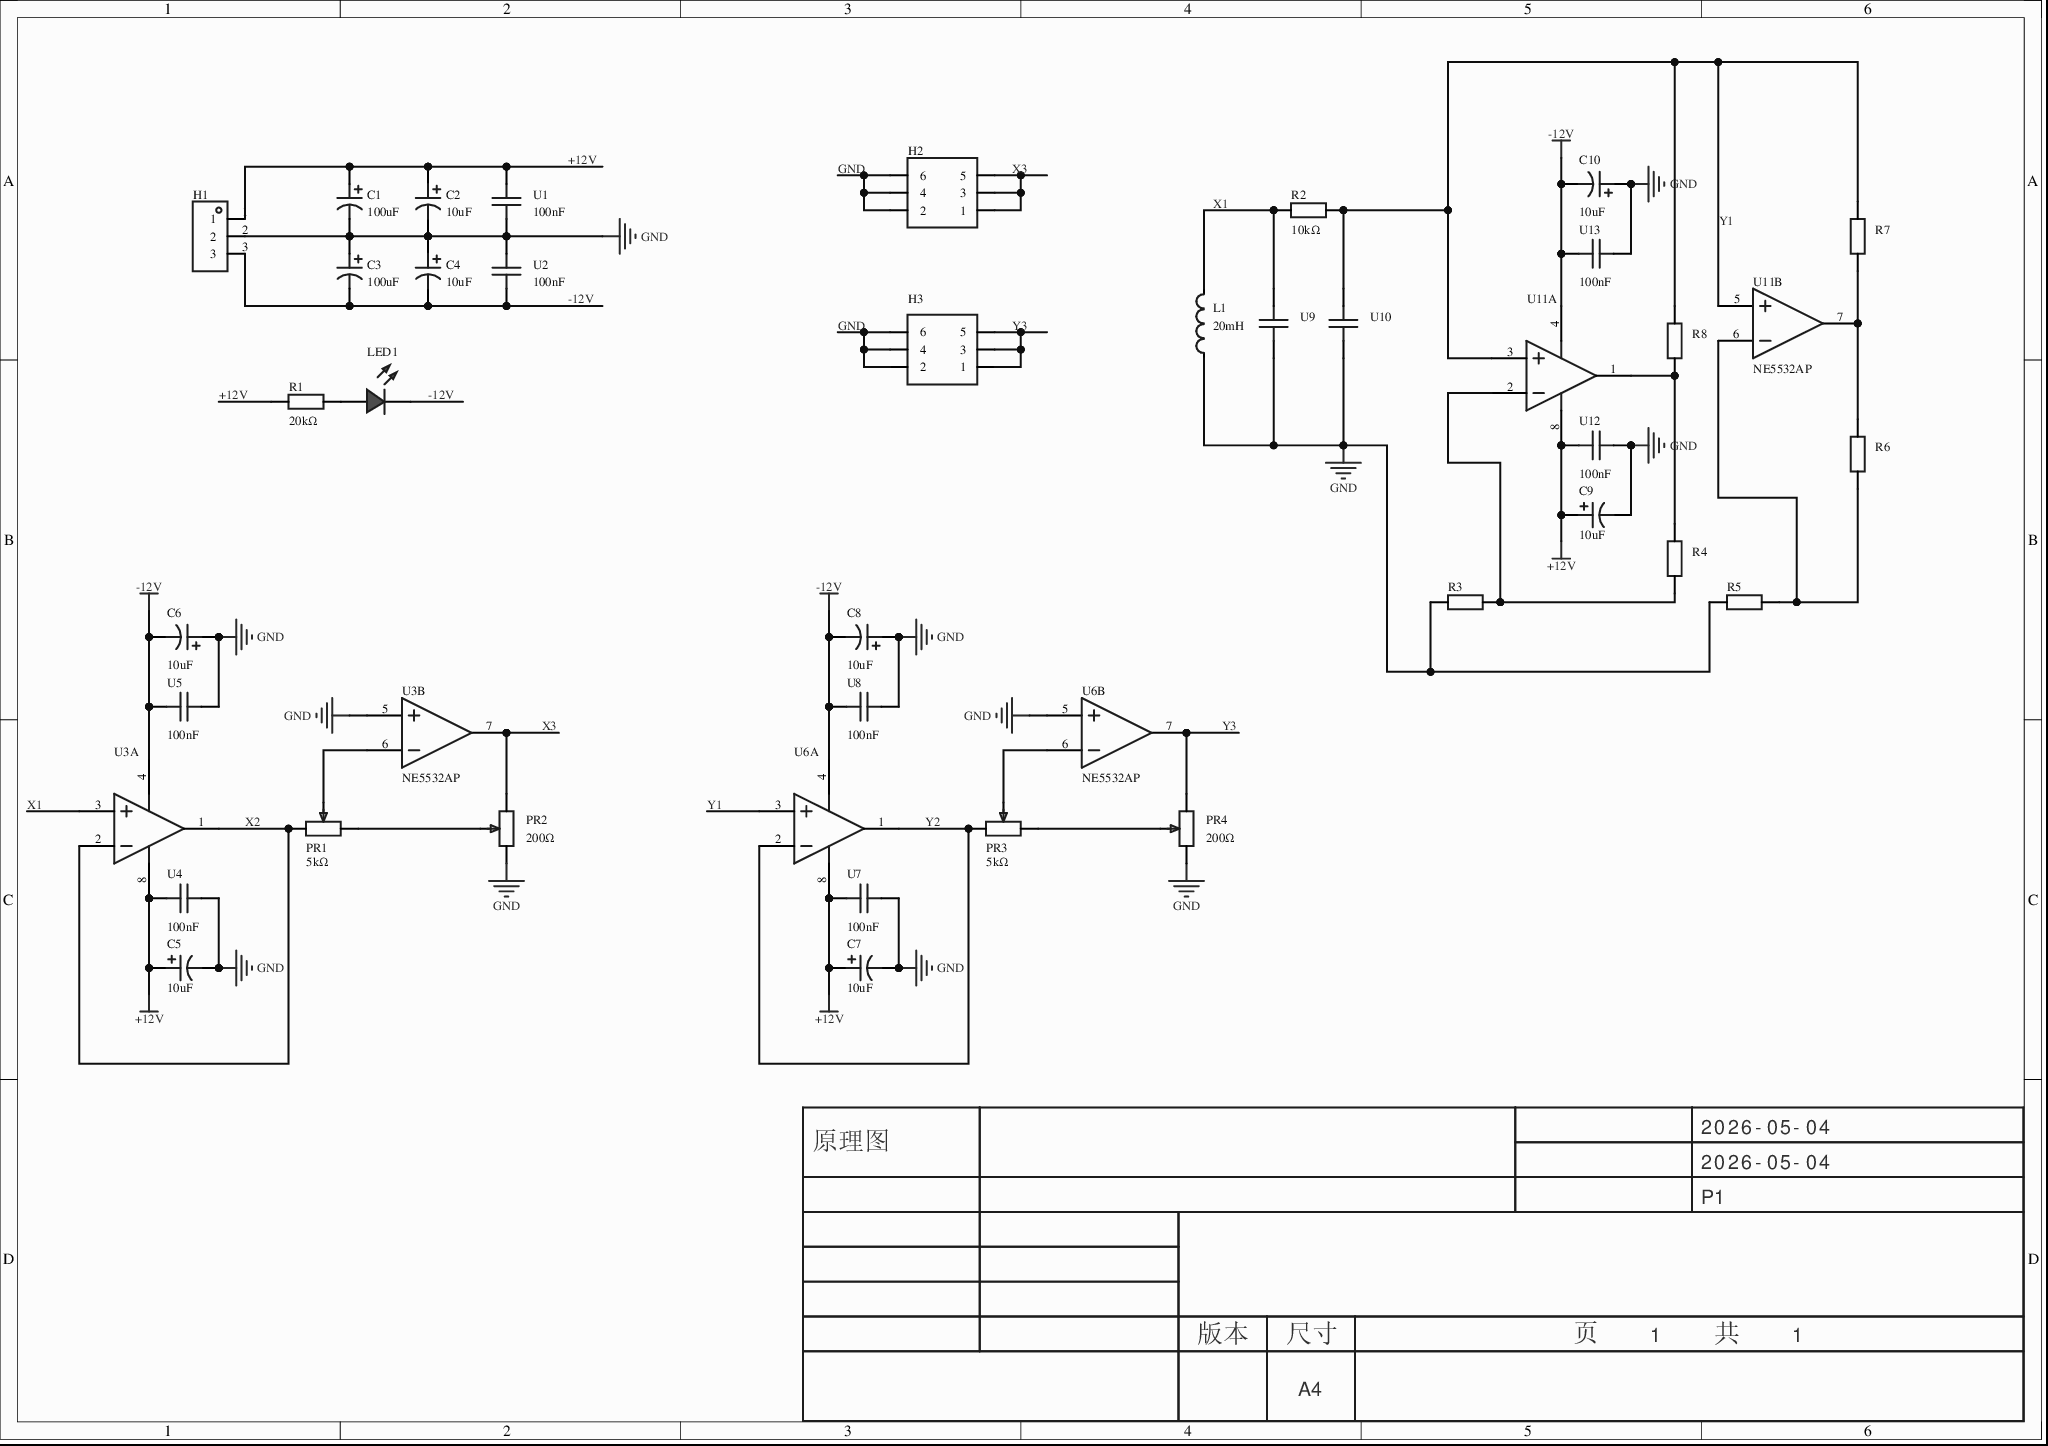
[diagram p0: MISC51743-3.schdoc]
# Altium project MISC51743-2.PrjPcb
1 sheet, 40 parts. Net scope: global (net labels, ports and power ports of the same name join across sheets).
Board file: MISC51743.pcbdoc

## Sheet MISC51743-3.schdoc
size 297 x 209 mm; Version: V1.0; @Project Name: MISC51743; @Update Date: 2026-05-04; @Create Date: 2026-05-04; @Board Name: MISC51743; @Create Time: 17:21:46; @Page Count: 1; @Page No: 1; @Schematic Name: MISC51743; @Update Time: 17:21:46; Size: A4

### Parts
C1  100uF  [CAP-TH_BD8.0-P3.50-D0.6-FD_1]
C2  10uF  [CAP-TH_BD5.0-P2.00-D0.8-FD-10UF50VC110GL]
C3  100uF  [CAP-TH_BD8.0-P3.50-D0.6-FD_1]
C4  10uF  [CAP-TH_BD5.0-P2.00-D0.8-FD-10UF50VC110GL]
C5  10uF  [CAP-TH_BD5.0-P2.00-D0.8-FD-10UF50VC110GL]
C6  10uF  [CAP-TH_BD5.0-P2.00-D0.8-FD-10UF50VC110GL]
C7  10uF  [CAP-TH_BD5.0-P2.00-D0.8-FD-10UF50VC110GL]
C8  10uF  [CAP-TH_BD5.0-P2.00-D0.8-FD-10UF50VC110GL]
C9  10uF  [CAP-TH_BD5.0-P2.00-D0.8-FD-10UF50VC110GL]
C10  10uF  [CAP-TH_BD5.0-P2.00-D0.8-FD-10UF50VC110GL]
H1  (no value)  [HDR-TH_3P-P2.54-V-M]
H2  (no value)  [HDR-TH_6P-P2.54-V-F-R2-C3-S2.54]
H3  (no value)  [HDR-TH_6P-P2.54-V-F-R2-C3-S2.54]
L1  20mH  [L0603]
LED1  (no value)  [LED_TH-3mm]
PR1  5kΩ  [R_3296]
PR2  200Ω  [R_3296]
PR3  5kΩ  [R_3296]
PR4  200Ω  [R_3296]
R1  20kΩ  [Res_1/8W]
R2  10kΩ  [Res_1/8W]
R3  10kΩ  [Res_1/8W]  (value not drawn)
R4  10kΩ  [Res_1/8W]  (value not drawn)
R5  10kΩ  [Res_1/8W]  (value not drawn)
R6  10kΩ  [Res_1/8W]  (value not drawn)
R7  10kΩ  [Res_1/8W]  (value not drawn)
R8  10kΩ  [Res_1/8W]  (value not drawn)
U1  100nF  [CAP-TH_L5.0-W2.5-P5.00-D1.0]
U2  100nF  [CAP-TH_L5.0-W2.5-P5.00-D1.0]
U3  NE5532AP  [PDIP-8_L9.6-W6.4-P2.54-LS7.6-BL]  (value not drawn)  (parts A,B of 2)
U4  100nF  [CAP-TH_L5.0-W2.5-P5.00-D1.0]
U5  100nF  [CAP-TH_L5.0-W2.5-P5.00-D1.0]
U6  NE5532AP  [PDIP-8_L9.6-W6.4-P2.54-LS7.6-BL]  (value not drawn)  (parts A,B of 2)
U7  100nF  [CAP-TH_L5.0-W2.5-P5.00-D1.0]
U8  100nF  [CAP-TH_L5.0-W2.5-P5.00-D1.0]
U9  100nF  [CAP-TH_L5.0-W2.5-P5.00-D1.0]  (value not drawn)
U10  100nF  [CAP-TH_L5.0-W2.5-P5.00-D1.0]  (value not drawn)
U11  NE5532AP  [PDIP-8_L9.6-W6.4-P2.54-LS7.6-BL]  (value not drawn)  (parts A,B of 2)
U12  100nF  [CAP-TH_L5.0-W2.5-P5.00-D1.0]
U13  100nF  [CAP-TH_L5.0-W2.5-P5.00-D1.0]

### Nets
+12V: C1.1 C2.1 C5.1 C7.1 C9.1 H1.1 R1.1 U1.1 U3.8(V+) U4.2 U6.8(V+) U7.2 U11.8(V+) U12.2
-12V: C3.2 C4.2 C6.2 C8.2 C10.2 H1.3 LED1.2(A) U2.2 U3.4(V-) U5.2 U6.4(V-) U8.2 U11.4(V-) U13.2
GND: C1.2 C2.2 C3.1 C4.1 C5.2 C6.1 C7.2 C8.1 C9.2 C10.1 H1.2 H2.2 H2.4 H2.6 H3.2 H3.4 H3.6 L1.1 PR2.3 PR4.3 R3.1 R5.1 U1.2 U2.1 U3.5(IN_B+) U4.1 U5.1 U6.5(IN_B+) U7.1 U8.1 U9.2 U10.2 U12.1 U13.1
X1: L1.2 R2.1 U3.3(IN_A+) U9.1
X2: PR1.3 U3.1(OUT_A) U3.2(IN_A-)
X3: H2.1 H2.3 H2.5 PR2.1 U3.7(OUT_B)
Y1: R2.2 R7.2 R8.2 U6.3(IN_A+) U10.1 U11.3(IN_A+) U11.5(IN_B+)
Y2: PR3.3 U6.1(OUT_A) U6.2(IN_A-)
Y3: H3.1 H3.3 H3.5 PR4.1 U6.7(OUT_B)
NetLED1_1: LED1.1(C) R1.2
NetPR1_1: PR1.1 PR2.2
NetPR1_2: PR1.2 U3.6(IN_B-)
NetPR3_1: PR3.1 PR4.2
NetPR3_2: PR3.2 U6.6(IN_B-)
NetR3_2: R3.2 R4.1 U11.2(IN_A-)
NetR4_2: R4.2 R8.1 U11.1(OUT_A)
NetR5_2: R5.2 R6.1 U11.6(IN_B-)
NetR6_2: R6.2 R7.1 U11.7(OUT_B)

### Notes on the sheet
- 2026-05-04
- 原理图
- P1
- 版本
- 尺寸
- A4
- 页    1    共    1

### Library data of the parts
C1 C3 = 100uF: Symbol: 100UF_C9900016884; AddInBom: yes; ModelId: 5fc21599cab34df2ad7753b19b2f52860819f05c4eef4c71ace90d822a990e87; ModelTransform: 315.365,314.914,0,0,0,0,0,0,-196.85; Device: 100uF; LCSC Part Name: 100uF; SupplierPart: C9900016884; ManufacturerPart: 100uF; Supplier Footprint: CAP-TH_BD8.0-P3.50-D1.0-FD; JLCPCB Part Class: Extended Part; Supplier: LCSC; ConvertToPcb: yes; FootprintName: CAP-TH_BD8.0-P3.50-D0.6-FD_1; ModelName: CAP-TH_BD8.0-P3.50-D0.6-FD_1
C2 C4-C10 = 10UF50VC110GL: 容值:10uF;精度:±20%;额定电压:50V;纹波电流:120mA@100KHz;等效串联电阻(ESR):1.6Ω;; Manufacturer: Econd(米朗电子); AddInBom: yes; Tolerance: ±20%; Voltage Rating: 50V; Equivalent Series Resistance(ESR): 1.6Ω; Pin Spacing: 2mm; Lifetime: 5000hrs@105℃; Symbol: 10UF50VC110GL; Device: 10UF50VC110GL; LCSC Part Name: 10uF ±20% 50V; SupplierPart: C46867109; ManufacturerPart: 10UF50VC110GL; Supplier Footprint: 插件,D5xL11mm; JLCPCB Part Class: Extended Part; Datasheet: https://item.szlcsc.com/datasheet/10UF50VC110GL/49031974.html; Supplier: LCSC; ConvertToPcb: yes; FootprintName: CAP-TH_BD5.0-P2.00-D0.8-FD-10UF50VC110GL; Value: 10uF; Ripple Current: 120mA@100KHz; Diameter: 5mm; Height - Seated (Max): 11mm; Operating Temperature: -40℃~+105℃
H1 = HDR-M_2.54_1x3P: AddInBom: yes; ModelId: bb473b6d38ff42a99216a4fcdbdcc4cb0819f05c4eef4c71ace90d822a990e87; ModelName: HDR-TH_3P-P2.54-M-LI-1X3P; ModelTransform: 300.03877,100,0,0,0,0,0,0,-118.11; Symbol: HDR-M_2.54_1x3P; Device: HDR-M_2.54_1x3P; ConvertToPcb: yes; FootprintName: HDR-TH_3P-P2.54-V-M; SupplierPart: C2937625; Supplier Footprint: 插件
H2 H3 = HDR-F_2.54_2x3: Symbol: HDR-F-2.54_2x3; ConvertToPcb: yes; ModelId: 6dbaf143e10146ae9674d03402f6f9fb0819f05c4eef4c71ace90d822a990e87; ModelName: HDR-TH_6P-P2.54-F-LI-2X3P; ModelTransform: 315.7474,196.85,0,0,0,0,0,0,-125.984; Device: HDR-F_2.54_2x3; AddInBom: yes; SupplierPart: C92272; Supplier Footprint: 插件; FootprintName: HDR-TH_6P-P2.54-V-F-R2-C3-S2.54
L1 = L_0603: Symbol: SDFL1608S100KTF; AddInBom: yes; ModelId: 2bc5ec593d464d6ba9807aec0b5673c20819f05c4eef4c71ace90d822a990e87; ModelName: L0603_L1.6-W0.8-H0.5_BEAD; ModelTransform: 62.992,31.496,0,180,0,0,0.094,0.629,0; Device: L_0603; Value: 20mH; Supplier Footprint: L0603; ConvertToPcb: yes; FootprintName: L0603
LED1 = LED_TH-R_3mm: ConvertToPcb: yes; ModelId: a497c992633541038a38947cdc58012f0819f05c4eef4c71ace90d822a990e87; ModelName: LED-TH-3mm_R; ModelTransform: 141.274,153.327,0,0,0,0,-5.984,0,-137.795; Symbol: LED_TH-R; Device: LED_TH-R_3mm; AddInBom: yes; FootprintName: LED_TH-3mm; Supplier Footprint: 插件
PR1-PR4 = R_3296: ConvertToPcb: yes; ModelId: b182808559bb43bda9e7de64b64134cb0819f05c4eef4c71ace90d822a990e87; ModelName: 3296W; ModelTransform: 373.98,188.96,590.49,180,0,0,0,0,-140; Symbol: R_3296; Device: R_3296; AddInBom: yes; Supplier Footprint: 直插; FootprintName: R_3296
  PR1 PR3: Value: 5kΩ
  PR2 PR4: Value: 200Ω
R1-R8 = Res_AXIAL-1/8W: Symbol: 电阻; ConvertToPcb: yes; ModelId: b2b5ae7ae4c642178fe0039925c86a3f0819f05c4eef4c71ace90d822a990e87; ModelName: RES-TH_BD1.8-L3.2-P7.20-D0.4; ModelTransform: 282.86,66.88,253.09,0,0,0,0,0,-191; Device: Res_AXIAL-1/8W; AddInBom: yes; Supplier Footprint: 轴向引线; FootprintName: Res_1/8W
  R1: Value: 20kΩ
  R2-R8: Value: 10kΩ
U1 U2 U4 U5 U7-U10 U12 U13 = 100nF: Symbol: 100NF_C9900015256; AddInBom: yes; ModelId: 08e3d7481fc7486bb1b263873f51e1e10819f05c4eef4c71ace90d822a990e87; ModelName: CAP-TH_BD5.0-W2.5-P5.08; ModelTransform: 224.652,98.425,0,0,0,0,-0.005,0,-137.795; Device: 100nF; LCSC Part Name: 100nF; SupplierPart: C9900015256; ManufacturerPart: 100nF; Supplier Footprint: CAP-TH_L5.0-W2.5-P5.00-D1.0; JLCPCB Part Class: Extended Part; Supplier: LCSC; ConvertToPcb: yes; FootprintName: CAP-TH_L5.0-W2.5-P5.00-D1.0
U3 U6 U11 = NE5532AP: NE5532A 适用于音频应用的双通道、30V、10MHz、低噪声 (6nV/√Hz) 运算放大器; Manufacturer: TI(德州仪器); Relevance: []; AddInBom: yes; ModelId: 5dc2af053da0476fab11ee64b9a10a940819f05c4eef4c71ace90d822a990e87; ModelName: PDIP-8_L9.6-W6.4-P2.54-LS7.62-BL; ModelTransform: 377.952,309.842,0,0,0,0,0,0,-137.795; Symbol: NE5532AP; Device: NE5532AP; LCSC Part Name: NE5532AP; SupplierPart: C353150; ManufacturerPart: NE5532AP; Supplier Footprint: PDIP-8; JLCPCB Part Class: Extended Part; Datasheet: https://www.ti.com/cn/lit/gpn/sa5532a; Supplier: LCSC; ConvertToPcb: yes; FootprintName: PDIP-8_L9.6-W6.4-P2.54-LS7.6-BL